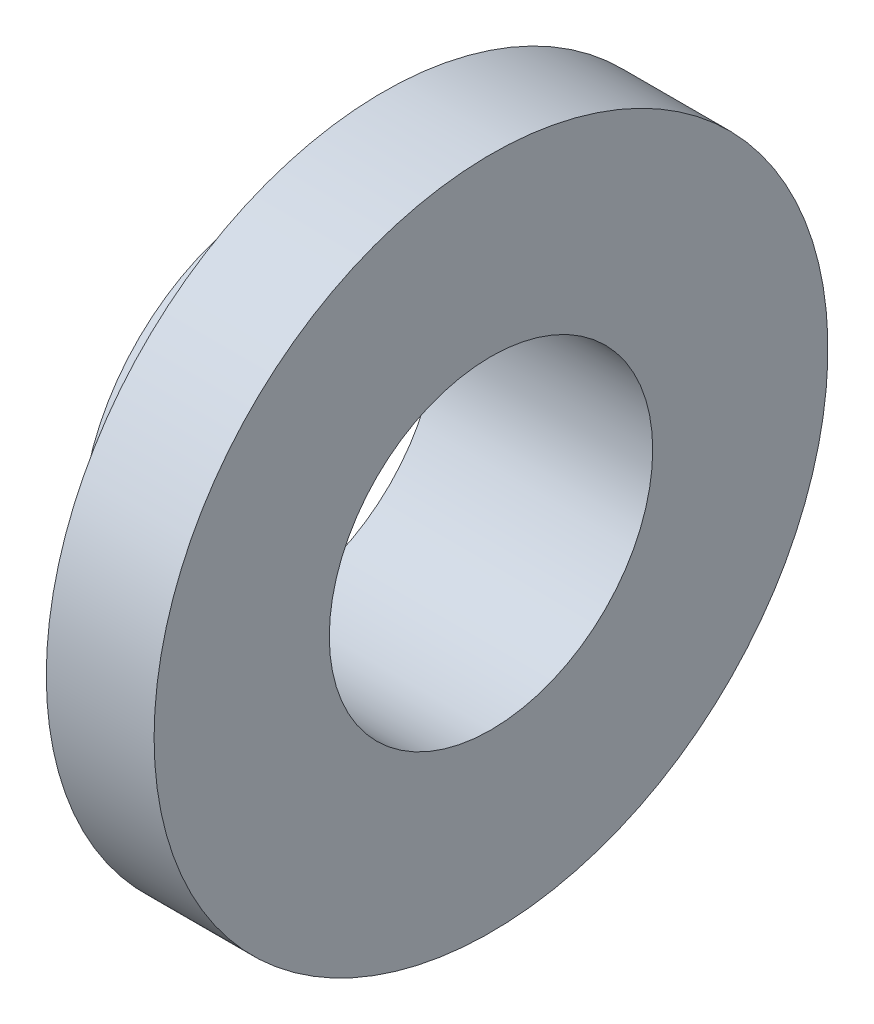
from build123d import *


with BuildPart() as part:
    # Sketch1 → Revolve1 (revolve)
    with BuildSketch(Plane.XY, mode=Mode.PRIVATE) as revolve1_sk:
        Polygon((0, -30), (0, -36), (20, -36), (20, -62.5), (40, -62.5), (40, -30), align=None)
    revolve(revolve1_sk.sketch.rotate(Axis((0, 0, 0), (1, 0, 0)), 270), axis=Axis((0, 0, 0), (1, 0, 0)))


solid = part.part
